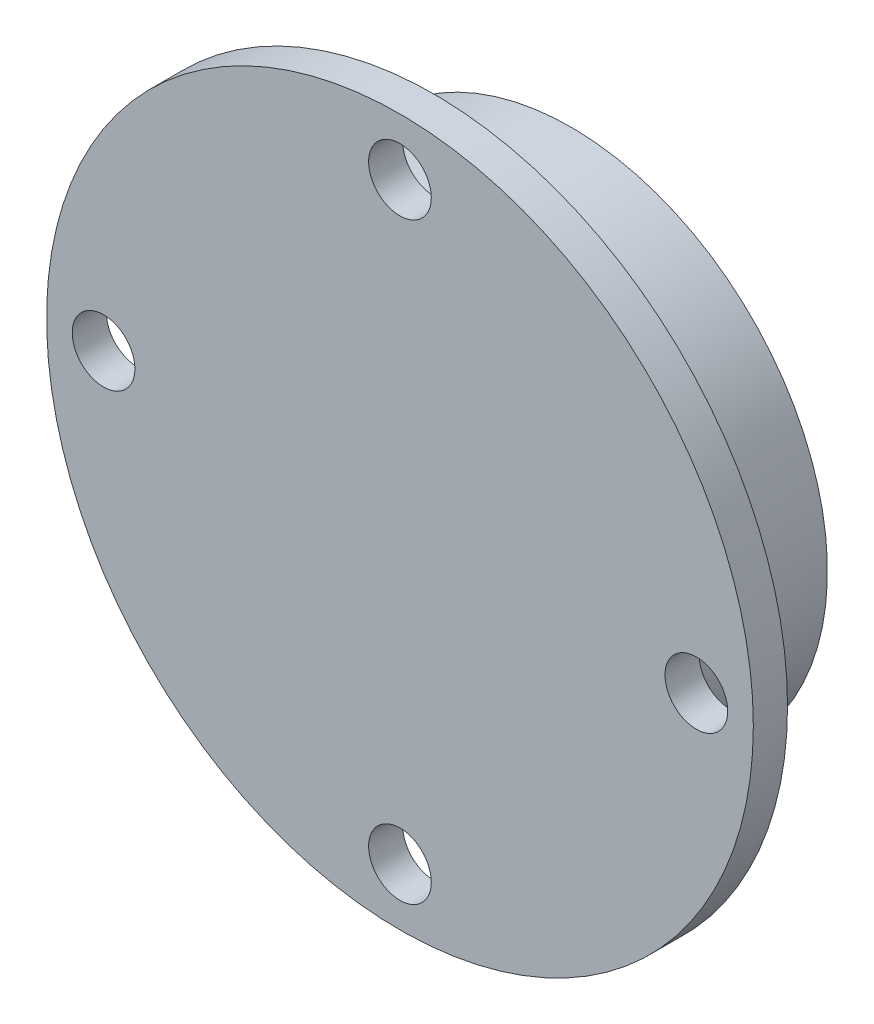
from build123d import *

# Parameters (mm, degrees)
SKETCH2_R           = 31
BOSS_EXTRUDE1_DEPTH = 3
SKETCH3_R           = 22.5
BOSS_EXTRUDE2_DEPTH = 12
SKETCH4_R           = 17.5
CUT_EXTRUDE1_DEPTH  = 9
SKETCH6_R           = 2.75
CUT_EXTRUDE2_DEPTH  = 12


with BuildPart() as part:
    # Sketch2 → Boss-Extrude1 (new body)
    with BuildSketch(Plane.XY.offset(-694.189912682)):
        with Locations((-50, 0)):
            Circle(SKETCH2_R)
    extrude(amount=BOSS_EXTRUDE1_DEPTH)

    # Sketch3 → Boss-Extrude2 (add)
    with BuildSketch(Plane(origin=(0, 0, -694.189912682), x_dir=(-1, 0, 0), z_dir=(0, 0, -1))):
        with Locations((50, 0)):
            Circle(SKETCH3_R)
    extrude(amount=BOSS_EXTRUDE2_DEPTH)

    # Sketch4 → Cut-Extrude1 (cut)
    with BuildSketch(Plane(origin=(0, 0, -706.189912682), x_dir=(-1, 0, 0), z_dir=(0, 0, -1))):
        with Locations((50, 0)):
            Circle(SKETCH4_R)
    extrude(amount=-CUT_EXTRUDE1_DEPTH, mode=Mode.SUBTRACT)

    # Sketch6 → Cut-Extrude2 (cut)
    with BuildSketch(Plane.XY.offset(-691.189912682)):
        with Locations((-50, 26)):
            Circle(SKETCH6_R)
        with Locations((-24, 0)):
            Circle(SKETCH6_R)
        with Locations((-50, -26)):
            Circle(SKETCH6_R)
        with Locations((-76, 0)):
            Circle(SKETCH6_R)
    extrude(amount=-CUT_EXTRUDE2_DEPTH, mode=Mode.SUBTRACT)


solid = part.part
